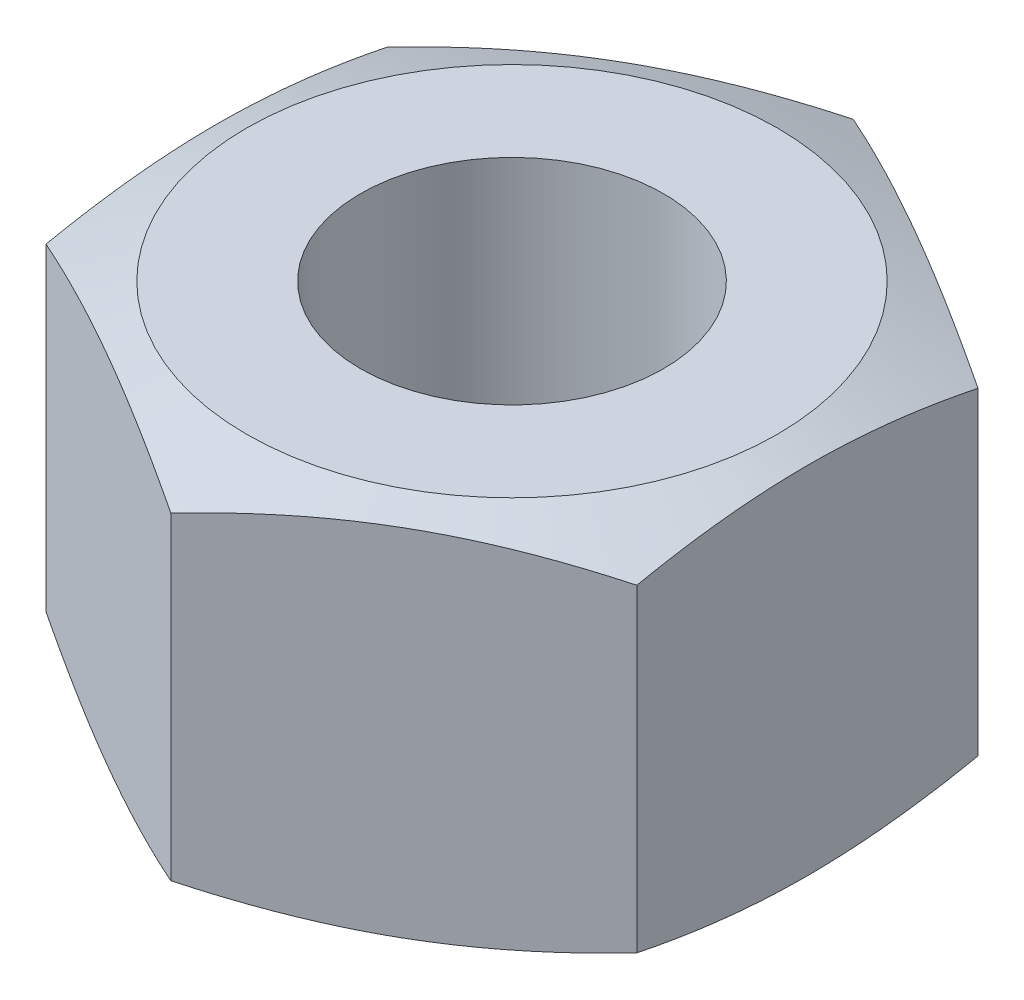
SolidWorks part; units mm, degrees
ref_plane "前视基准面" through (0, 0, 0) normal (0, 0, 1) x (1, 0, 0)
ref_plane "上视基准面" through (0, 0, 0) normal (0, 1, 0) x (1, 0, 0)
ref_plane "右视基准面" through (0, 0, 0) normal (1, 0, 0) x (0, 0, -1)
sketch "草图1" plane through (0, 0, 0) normal (0, 1, 0) x (1, 0, 0)
  line L1 (0, 22.5) -> (-19.4856, 11.25)
  line L2 (-19.4856, 11.25) -> (-19.4856, -11.25)
  line L3 (-19.4856, -11.25) -> (0, -22.5)
  line L4 (0, -22.5) -> (19.4856, -11.25)
  line L5 (19.4856, -11.25) -> (19.4856, 11.25)
  line L6 (19.4856, 11.25) -> (0, 22.5)
  circle A0 centre (0, 0) radius 19.4856 construction
  circle A1 centre (0, 0) radius 10
  dimension "D1" = 20
  dimension "D2" = 45
extrude "凸台-拉伸1" add sketch "草图1" along normal mid plane 25
sketch "草图2" plane through (0, 0, 0) normal (1, 0, 0) x (0, 0, -1)
  line L0 (0, 32.4997) -> (0, -7.2502) construction
  line L1 (-22.5, 10.5) -> (-22.5, 12.5)
  line L2 (-22.5, 12.5) -> (-11.25, 12.5) construction
  line L3 (-22.5, 12.5) -> (-17.5, 12.5)
  arc A0 (-17.5, 12.5) -> (-22.5, 10.5) centre (72.8423, -220.6057) ccw
  dimension "D1" = 500
  dimension "D2" = 5
  dimension "D3" = 2
revolve "切除-旋转1" cut sketch "草图2" angle 360 about L0
mirror "镜向1" about plane through (0, 0, 0) normal (0, 1, 0) of "切除-旋转1"
